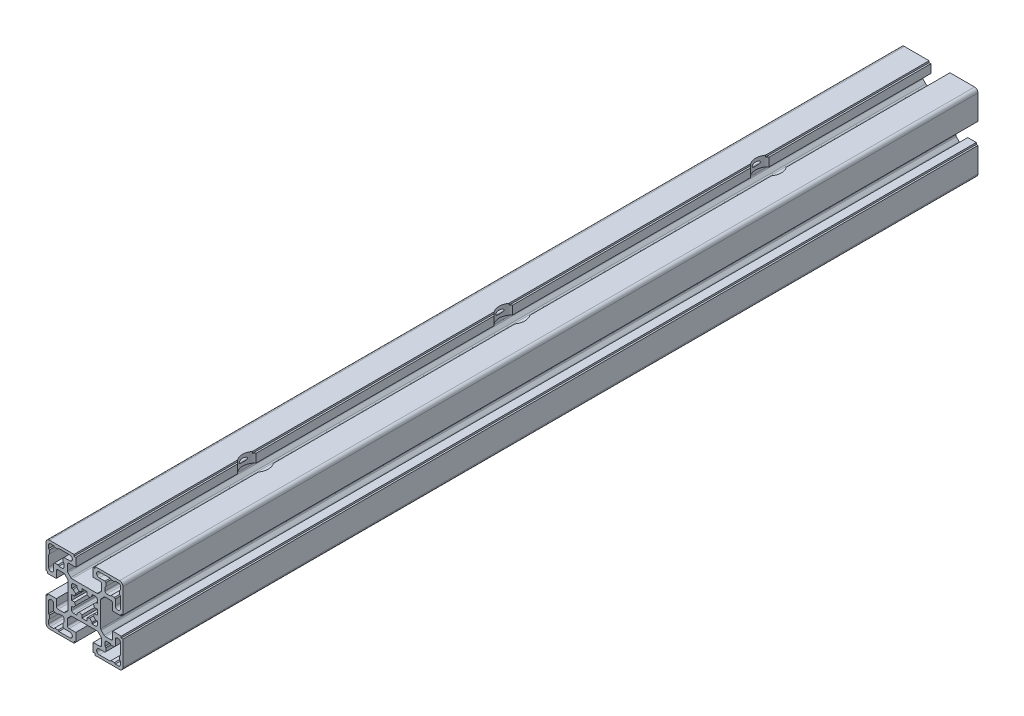
SolidWorks part; units mm, degrees
material "1.11.45.045045.04"
ref_plane "前视基准面" through (0, 0, 0) normal (0, 0, 1) x (1, 0, 0)
ref_plane "上视基准面" through (0, 0, 0) normal (0, 1, 0) x (1, 0, 0)
ref_plane "右视基准面" through (0, 0, 0) normal (1, 0, 0) x (0, 0, -1)
sketch "草图1" plane through (0, 0, 0) normal (0, 0, 1) x (1, 0, 0)
  line L0 (30.535, 44.0271) -> (29.0823, 45.4798)
  line L1 (31.4137, 44.0271) -> (30.535, 44.0271)
  line L2 (31.4137, 42.0271) -> (31.4137, 44.0271)
  line L3 (28.4137, 41.0271) -> (30.4137, 41.0271)
  line L4 (28.4137, 41.9058) -> (28.4137, 41.0271)
  line L5 (26.961, 43.3585) -> (28.4137, 41.9058)
  line L6 (25.4137, 41.0271) -> (25.4137, 42.7176)
  line L7 (22.4137, 41.0271) -> (25.4137, 41.0271)
  line L8 (22.4137, 42.7176) -> (22.4137, 41.0271)
  line L9 (19.4137, 41.9058) -> (20.8664, 43.3585)
  line L10 (19.4137, 41.0271) -> (19.4137, 41.9058)
  line L11 (17.4137, 41.0271) -> (19.4137, 41.0271)
  line L12 (16.4137, 44.0271) -> (16.4137, 42.0271)
  line L13 (17.2924, 44.0271) -> (16.4137, 44.0271)
  line L14 (18.7451, 45.4798) -> (17.2924, 44.0271)
  line L15 (16.4137, 47.0271) -> (18.1042, 47.0271)
  line L16 (16.4137, 50.0271) -> (16.4137, 47.0271)
  line L17 (18.1042, 50.0271) -> (16.4137, 50.0271)
  line L18 (17.2924, 53.0271) -> (18.7451, 51.5744)
  line L19 (16.4137, 53.0271) -> (17.2924, 53.0271)
  line L20 (16.4137, 55.0271) -> (16.4137, 53.0271)
  line L21 (19.4137, 56.0271) -> (17.4137, 56.0271)
  line L22 (19.4137, 55.1484) -> (19.4137, 56.0271)
  line L23 (20.8664, 53.6957) -> (19.4137, 55.1484)
  line L24 (22.4137, 56.0271) -> (22.4137, 54.3366)
  line L25 (25.4137, 56.0271) -> (22.4137, 56.0271)
  line L26 (25.4137, 54.3366) -> (25.4137, 56.0271)
  line L27 (28.4137, 55.1484) -> (26.961, 53.6957)
  line L28 (28.4137, 56.0271) -> (28.4137, 55.1484)
  line L29 (30.4137, 56.0271) -> (28.4137, 56.0271)
  line L30 (31.4137, 53.0271) -> (31.4137, 55.0271)
  line L31 (30.535, 53.0271) -> (31.4137, 53.0271)
  line L32 (29.0823, 51.5744) -> (30.535, 53.0271)
  line L33 (31.4137, 50.0271) -> (29.7232, 50.0271)
  line L34 (31.4137, 47.0271) -> (31.4137, 50.0271)
  line L35 (29.7232, 47.0271) -> (31.4137, 47.0271)
  line L36 (11.4137, 66.0271) -> (11.9137, 66.5271)
  line L37 (11.4137, 64.0271) -> (11.4137, 66.0271)
  line L38 (11.9137, 63.5271) -> (11.4137, 64.0271)
  line L39 (11.9137, 61.5271) -> (11.9137, 63.5271)
  line L40 (8.9137, 60.5271) -> (10.9137, 60.5271)
  line L41 (8.4137, 61.0271) -> (8.9137, 60.5271)
  line L42 (6.4137, 61.0271) -> (8.4137, 61.0271)
  line L43 (5.9137, 60.5271) -> (6.4137, 61.0271)
  line L44 (5.9137, 57.1271) -> (5.9137, 60.5271)
  line L45 (2.9137, 63.5271) -> (2.9137, 57.1271)
  line L46 (3.4137, 64.0271) -> (2.9137, 63.5271)
  line L47 (3.4137, 66.0271) -> (3.4137, 64.0271)
  line L48 (2.9137, 66.5271) -> (3.4137, 66.0271)
  line L49 (2.9137, 68.5271) -> (2.9137, 66.5271)
  line L50 (5.9137, 69.5271) -> (3.9137, 69.5271)
  line L51 (6.4137, 69.0271) -> (5.9137, 69.5271)
  line L52 (8.4137, 69.0271) -> (6.4137, 69.0271)
  line L53 (8.9137, 69.5271) -> (8.4137, 69.0271)
  line L54 (15.3137, 69.5271) -> (8.9137, 69.5271)
  line L55 (11.9137, 66.5271) -> (15.3137, 66.5271)
  line L56 (11.9137, 30.5271) -> (11.4137, 31.0271)
  line L57 (15.3137, 30.5271) -> (11.9137, 30.5271)
  line L58 (8.9137, 27.5271) -> (15.3137, 27.5271)
  line L59 (8.4137, 28.0271) -> (8.9137, 27.5271)
  line L60 (6.4137, 28.0271) -> (8.4137, 28.0271)
  line L61 (5.9137, 27.5271) -> (6.4137, 28.0271)
  line L62 (3.9137, 27.5271) -> (5.9137, 27.5271)
  line L63 (2.9137, 30.5271) -> (2.9137, 28.5271)
  line L64 (3.4137, 31.0271) -> (2.9137, 30.5271)
  line L65 (3.4137, 33.0271) -> (3.4137, 31.0271)
  line L66 (2.9137, 33.5271) -> (3.4137, 33.0271)
  line L67 (2.9137, 39.9271) -> (2.9137, 33.5271)
  line L68 (5.9137, 36.5271) -> (5.9137, 39.9271)
  line L69 (6.4137, 36.0271) -> (5.9137, 36.5271)
  line L70 (8.4137, 36.0271) -> (6.4137, 36.0271)
  line L71 (8.9137, 36.5271) -> (8.4137, 36.0271)
  line L72 (10.9137, 36.5271) -> (8.9137, 36.5271)
  line L73 (11.9137, 33.5271) -> (11.9137, 35.5271)
  line L74 (11.4137, 33.0271) -> (11.9137, 33.5271)
  line L75 (11.4137, 31.0271) -> (11.4137, 33.0271)
  line L76 (41.9137, 36.5271) -> (41.4137, 36.0271)
  line L77 (41.9137, 39.9271) -> (41.9137, 36.5271)
  line L78 (44.9137, 33.5271) -> (44.9137, 39.9271)
  line L79 (44.4137, 33.0271) -> (44.9137, 33.5271)
  line L80 (44.4137, 31.0271) -> (44.4137, 33.0271)
  line L81 (44.9137, 30.5271) -> (44.4137, 31.0271)
  line L82 (44.9137, 28.5271) -> (44.9137, 30.5271)
  line L83 (41.9137, 27.5271) -> (43.9137, 27.5271)
  line L84 (41.4137, 28.0271) -> (41.9137, 27.5271)
  line L85 (39.4137, 28.0271) -> (41.4137, 28.0271)
  line L86 (38.9137, 27.5271) -> (39.4137, 28.0271)
  line L87 (32.5137, 27.5271) -> (38.9137, 27.5271)
  line L88 (35.9137, 30.5271) -> (32.5137, 30.5271)
  line L89 (36.4137, 31.0271) -> (35.9137, 30.5271)
  line L90 (36.4137, 33.0271) -> (36.4137, 31.0271)
  line L91 (35.9137, 33.5271) -> (36.4137, 33.0271)
  line L92 (35.9137, 35.5271) -> (35.9137, 33.5271)
  line L93 (38.9137, 36.5271) -> (36.9137, 36.5271)
  line L94 (39.4137, 36.0271) -> (38.9137, 36.5271)
  line L95 (41.4137, 36.0271) -> (39.4137, 36.0271)
  line L96 (35.9137, 66.5271) -> (36.4137, 66.0271)
  line L97 (32.5137, 66.5271) -> (35.9137, 66.5271)
  line L98 (38.9137, 69.5271) -> (32.5137, 69.5271)
  line L99 (39.4137, 69.0271) -> (38.9137, 69.5271)
  line L100 (41.4137, 69.0271) -> (39.4137, 69.0271)
  line L101 (41.9137, 69.5271) -> (41.4137, 69.0271)
  line L102 (43.9137, 69.5271) -> (41.9137, 69.5271)
  line L103 (44.9137, 66.5271) -> (44.9137, 68.5271)
  line L104 (44.4137, 66.0271) -> (44.9137, 66.5271)
  line L105 (44.4137, 64.0271) -> (44.4137, 66.0271)
  line L106 (44.9137, 63.5271) -> (44.4137, 64.0271)
  line L107 (44.9137, 57.1271) -> (44.9137, 63.5271)
  line L108 (41.9137, 60.5271) -> (41.9137, 57.1271)
  line L109 (41.4137, 61.0271) -> (41.9137, 60.5271)
  line L110 (39.4137, 61.0271) -> (41.4137, 61.0271)
  line L111 (38.9137, 60.5271) -> (39.4137, 61.0271)
  line L112 (36.9137, 60.5271) -> (38.9137, 60.5271)
  line L113 (35.9137, 63.5271) -> (35.9137, 61.5271)
  line L114 (36.4137, 64.0271) -> (35.9137, 63.5271)
  line L115 (36.4137, 66.0271) -> (36.4137, 64.0271)
  line L116 (33.7066, 40.502) -> (35.3886, 38.82)
  line L117 (33.4137, 55.8451) -> (33.4137, 41.2091)
  line L118 (35.3886, 58.2342) -> (33.7066, 56.5522)
  line L119 (39.4137, 58.5271) -> (36.0957, 58.5271)
  line L120 (40.4137, 53.6271) -> (40.4137, 57.5271)
  line L121 (45.4137, 53.6271) -> (40.4137, 53.6271)
  line L122 (45.4137, 54.6271) -> (45.4137, 53.6271)
  line L123 (46.4137, 54.6271) -> (45.4137, 54.6271)
  line L124 (46.4137, 69.0271) -> (46.4137, 54.6271)
  line L125 (30.0137, 71.0271) -> (44.4137, 71.0271)
  line L126 (30.0137, 70.0271) -> (30.0137, 71.0271)
  line L127 (29.0137, 70.0271) -> (30.0137, 70.0271)
  line L128 (29.0137, 65.0271) -> (29.0137, 70.0271)
  line L129 (32.9137, 65.0271) -> (29.0137, 65.0271)
  line L130 (33.9137, 60.7091) -> (33.9137, 64.0271)
  line L131 (31.9388, 58.32) -> (33.6208, 60.002)
  line L132 (16.5957, 58.0271) -> (31.2317, 58.0271)
  line L133 (14.2066, 60.002) -> (15.8886, 58.32)
  line L134 (13.9137, 64.0271) -> (13.9137, 60.7091)
  line L135 (18.8137, 65.0271) -> (14.9137, 65.0271)
  line L136 (18.8137, 70.0271) -> (18.8137, 65.0271)
  line L137 (17.8137, 70.0271) -> (18.8137, 70.0271)
  line L138 (17.8137, 71.0271) -> (17.8137, 70.0271)
  line L139 (3.4137, 71.0271) -> (17.8137, 71.0271)
  line L140 (1.4137, 54.6271) -> (1.4137, 69.0271)
  line L141 (2.4137, 54.6271) -> (1.4137, 54.6271)
  line L142 (2.4137, 53.6271) -> (2.4137, 54.6271)
  line L143 (7.4137, 53.6271) -> (2.4137, 53.6271)
  line L144 (7.4137, 57.5271) -> (7.4137, 53.6271)
  line L145 (11.7317, 58.5271) -> (8.4137, 58.5271)
  line L146 (14.1208, 56.5522) -> (12.4388, 58.2342)
  line L147 (14.4137, 41.2091) -> (14.4137, 55.8451)
  line L148 (12.4388, 38.82) -> (14.1208, 40.502)
  line L149 (8.4137, 38.5271) -> (11.7317, 38.5271)
  line L150 (7.4137, 43.4271) -> (7.4137, 39.5271)
  line L151 (2.4137, 43.4271) -> (7.4137, 43.4271)
  line L152 (2.4137, 42.4271) -> (2.4137, 43.4271)
  line L153 (1.4137, 42.4271) -> (2.4137, 42.4271)
  line L154 (1.4137, 28.0271) -> (1.4137, 42.4271)
  line L155 (17.8137, 26.0271) -> (3.4137, 26.0271)
  line L156 (17.8137, 27.0271) -> (17.8137, 26.0271)
  line L157 (18.8137, 27.0271) -> (17.8137, 27.0271)
  line L158 (18.8137, 32.0271) -> (18.8137, 27.0271)
  line L159 (14.9137, 32.0271) -> (18.8137, 32.0271)
  line L160 (13.9137, 36.3451) -> (13.9137, 33.0271)
  line L161 (15.8886, 38.7342) -> (14.2066, 37.0522)
  line L162 (31.2317, 39.0271) -> (16.5957, 39.0271)
  line L163 (33.6208, 37.0522) -> (31.9388, 38.7342)
  line L164 (33.9137, 33.0271) -> (33.9137, 36.3451)
  line L165 (29.0137, 32.0271) -> (32.9137, 32.0271)
  line L166 (29.0137, 27.0271) -> (29.0137, 32.0271)
  line L167 (30.0137, 27.0271) -> (29.0137, 27.0271)
  line L168 (30.0137, 26.0271) -> (30.0137, 27.0271)
  line L169 (44.4137, 26.0271) -> (30.0137, 26.0271)
  line L170 (46.4137, 42.4271) -> (46.4137, 28.0271)
  line L171 (45.4137, 42.4271) -> (46.4137, 42.4271)
  line L172 (45.4137, 43.4271) -> (45.4137, 42.4271)
  line L173 (40.4137, 43.4271) -> (45.4137, 43.4271)
  line L174 (40.4137, 39.5271) -> (40.4137, 43.4271)
  line L175 (36.0957, 38.5271) -> (39.4137, 38.5271)
  arc A0 (30.4137, 41.0271) -> (31.4137, 42.0271) centre (30.4137, 42.0271) ccw
  arc A1 (25.4137, 42.7176) -> (26.961, 43.3585) centre (23.9137, 48.5271) ccw
  arc A2 (20.8664, 43.3585) -> (22.4137, 42.7176) centre (23.9137, 48.5271) ccw
  arc A3 (16.4137, 42.0271) -> (17.4137, 41.0271) centre (17.4137, 42.0271) ccw
  arc A4 (18.1042, 47.0271) -> (18.7451, 45.4798) centre (23.9137, 48.5271) ccw
  arc A5 (18.7451, 51.5744) -> (18.1042, 50.0271) centre (23.9137, 48.5271) ccw
  arc A6 (17.4137, 56.0271) -> (16.4137, 55.0271) centre (17.4137, 55.0271) ccw
  arc A7 (22.4137, 54.3366) -> (20.8664, 53.6957) centre (23.9137, 48.5271) ccw
  arc A8 (26.961, 53.6957) -> (25.4137, 54.3366) centre (23.9137, 48.5271) ccw
  arc A9 (31.4137, 55.0271) -> (30.4137, 56.0271) centre (30.4137, 55.0271) ccw
  arc A10 (29.7232, 50.0271) -> (29.0823, 51.5744) centre (23.9137, 48.5271) ccw
  arc A11 (29.0823, 45.4798) -> (29.7232, 47.0271) centre (23.9137, 48.5271) ccw
  arc A12 (10.9137, 60.5271) -> (11.9137, 61.5271) centre (10.9137, 61.5271) ccw
  arc A13 (2.9137, 57.1271) -> (5.9137, 57.1271) centre (4.4137, 57.1271) ccw
  arc A14 (3.9137, 69.5271) -> (2.9137, 68.5271) centre (3.9137, 68.5271) ccw
  arc A15 (15.3137, 66.5271) -> (15.3137, 69.5271) centre (15.3137, 68.0271) ccw
  arc A16 (15.3137, 27.5271) -> (15.3137, 30.5271) centre (15.3137, 29.0271) ccw
  arc A17 (2.9137, 28.5271) -> (3.9137, 27.5271) centre (3.9137, 28.5271) ccw
  arc A18 (5.9137, 39.9271) -> (2.9137, 39.9271) centre (4.4137, 39.9271) ccw
  arc A19 (11.9137, 35.5271) -> (10.9137, 36.5271) centre (10.9137, 35.5271) ccw
  arc A20 (44.9137, 39.9271) -> (41.9137, 39.9271) centre (43.4137, 39.9271) ccw
  arc A21 (43.9137, 27.5271) -> (44.9137, 28.5271) centre (43.9137, 28.5271) ccw
  arc A22 (32.5137, 30.5271) -> (32.5137, 27.5271) centre (32.5137, 29.0271) ccw
  arc A23 (36.9137, 36.5271) -> (35.9137, 35.5271) centre (36.9137, 35.5271) ccw
  arc A24 (32.5137, 69.5271) -> (32.5137, 66.5271) centre (32.5137, 68.0271) ccw
  arc A25 (44.9137, 68.5271) -> (43.9137, 69.5271) centre (43.9137, 68.5271) ccw
  arc A26 (41.9137, 57.1271) -> (44.9137, 57.1271) centre (43.4137, 57.1271) ccw
  arc A27 (35.9137, 61.5271) -> (36.9137, 60.5271) centre (36.9137, 61.5271) ccw
  arc A28 (35.3886, 38.82) -> (36.0957, 38.5271) centre (36.0957, 39.5271) ccw
  arc A29 (33.4137, 41.2091) -> (33.7066, 40.502) centre (34.4137, 41.2091) ccw
  arc A30 (33.7066, 56.5522) -> (33.4137, 55.8451) centre (34.4137, 55.8451) ccw
  arc A31 (36.0957, 58.5271) -> (35.3886, 58.2342) centre (36.0957, 57.5271) ccw
  arc A32 (40.4137, 57.5271) -> (39.4137, 58.5271) centre (39.4137, 57.5271) ccw
  arc A33 (46.4137, 69.0271) -> (44.4137, 71.0271) centre (44.4137, 69.0271) ccw
  arc A34 (33.9137, 64.0271) -> (32.9137, 65.0271) centre (32.9137, 64.0271) ccw
  arc A35 (33.6208, 60.002) -> (33.9137, 60.7091) centre (32.9137, 60.7091) ccw
  arc A36 (31.2317, 58.0271) -> (31.9388, 58.32) centre (31.2317, 59.0271) ccw
  arc A37 (15.8886, 58.32) -> (16.5957, 58.0271) centre (16.5957, 59.0271) ccw
  arc A38 (13.9137, 60.7091) -> (14.2066, 60.002) centre (14.9137, 60.7091) ccw
  arc A39 (14.9137, 65.0271) -> (13.9137, 64.0271) centre (14.9137, 64.0271) ccw
  arc A40 (3.4137, 71.0271) -> (1.4137, 69.0271) centre (3.4137, 69.0271) ccw
  arc A41 (8.4137, 58.5271) -> (7.4137, 57.5271) centre (8.4137, 57.5271) ccw
  arc A42 (12.4388, 58.2342) -> (11.7317, 58.5271) centre (11.7317, 57.5271) ccw
  arc A43 (14.4137, 55.8451) -> (14.1208, 56.5522) centre (13.4137, 55.8451) ccw
  arc A44 (14.1208, 40.502) -> (14.4137, 41.2091) centre (13.4137, 41.2091) ccw
  arc A45 (11.7317, 38.5271) -> (12.4388, 38.82) centre (11.7317, 39.5271) ccw
  arc A46 (7.4137, 39.5271) -> (8.4137, 38.5271) centre (8.4137, 39.5271) ccw
  arc A47 (1.4137, 28.0271) -> (3.4137, 26.0271) centre (3.4137, 28.0271) ccw
  arc A48 (13.9137, 33.0271) -> (14.9137, 32.0271) centre (14.9137, 33.0271) ccw
  arc A49 (14.2066, 37.0522) -> (13.9137, 36.3451) centre (14.9137, 36.3451) ccw
  arc A50 (16.5957, 39.0271) -> (15.8886, 38.7342) centre (16.5957, 38.0271) ccw
  arc A51 (31.9388, 38.7342) -> (31.2317, 39.0271) centre (31.2317, 38.0271) ccw
  arc A52 (33.9137, 36.3451) -> (33.6208, 37.0522) centre (32.9137, 36.3451) ccw
  arc A53 (32.9137, 32.0271) -> (33.9137, 33.0271) centre (32.9137, 33.0271) ccw
  arc A54 (44.4137, 26.0271) -> (46.4137, 28.0271) centre (44.4137, 28.0271) ccw
  arc A55 (39.4137, 38.5271) -> (40.4137, 39.5271) centre (39.4137, 39.5271) ccw
extrude "拉伸1" add sketch "草图1" along normal blind 500
hole_wizard "打孔尺寸(%根据)内六角圆柱头螺钉的类型1" positions "草图3" profile "草图2" counterbore size "M8" standard "GB" end condition through all
sketch "草图3" plane through (0, 71.0271, 0) normal (0, 1, 0) x (1, 0, 0)
  line L0 (23.9137, 0) -> (23.9137, -500) construction
  line L1 (31.2317, 0) -> (16.5957, 0) construction
  line L2 (31.2317, -500) -> (16.5957, -500) construction
  point P0 (23.9137, -400)
  point P2 (23.9137, -250)
  point P4 (23.9137, -100)
  dimension "D1" = 100
  dimension "D2" = 100
sketch "草图2" plane through (23.9137, 71.0271, 400) normal (1, 0, 0) x (0, 0, 1)
  line L0 (0, 0) -> (0, 45)
  line L1 (0, 45) -> (5, 45)
  line L3 (5, 45) -> (5, 9)
  line L4 (5, 9) -> (7.5, 9)
  line L5 (7.5, 9) -> (7.5, 0)
  line L7 (7.5, 0) -> (0, 0)
  line L11 (0, -6.35) -> (0, 107.95) construction
  dimension "通孔孔直径" = 10
  dimension "通孔孔深度" = 45
  dimension "柱形沉头孔直径" = 15
  dimension "柱形沉头孔深度" = 9
